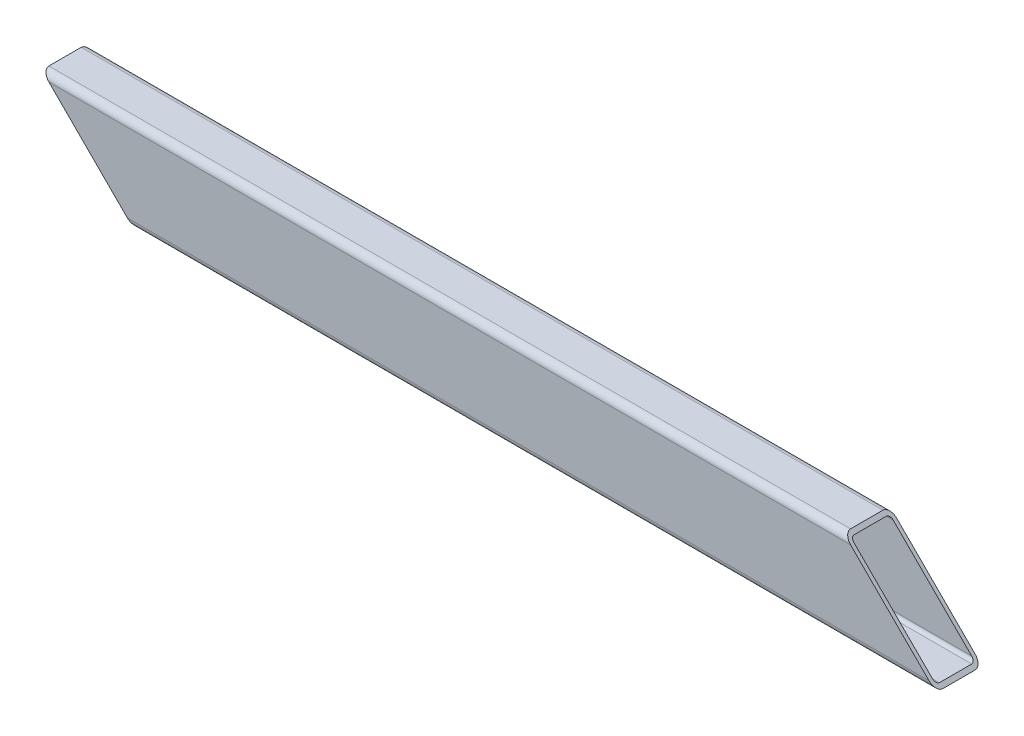
from build123d import *

# Parameters (mm, degrees)
COLD_FORMED_RECT_HOLLOW_SECTION_GB_T_672_DEPTH = 775
CUT_EXTRUDE1_DEPTH                             = 778.061773606


with BuildPart() as part:
    # Sketch1 → Cold-Formed Rect Hollow Section GB/T 6728-2002 80 X 40 X 3(1) (new body)
    with BuildSketch(Plane(origin=(0, 0, 0), x_dir=(0, 0, -1), z_dir=(1, 0, 0))):
        with BuildLine():
            Line((-14, -40), (14, -40))
            ThreePointArc((14, -40), (18.242640687, -38.242640687), (20, -34))
            Line((20, -34), (20, 34))
            ThreePointArc((20, 34), (18.242640687, 38.242640687), (14, 40))
            Line((14, 40), (-14, 40))
            ThreePointArc((-14, 40), (-18.242640687, 38.242640687), (-20, 34))
            Line((-20, 34), (-20, -34))
            ThreePointArc((-20, -34), (-18.242640687, -38.242640687), (-14, -40))
        make_face()
        with BuildLine():
            Line((-14, -37), (14, -37))
            ThreePointArc((14, -37), (16.121320344, -36.121320344), (17, -34))
            Line((17, -34), (17, 34))
            ThreePointArc((17, 34), (16.121320344, 36.121320344), (14, 37))
            Line((14, 37), (-14, 37))
            ThreePointArc((-14, 37), (-16.121320344, 36.121320344), (-17, 34))
            Line((-17, 34), (-17, -34))
            ThreePointArc((-17, -34), (-16.121320344, -36.121320344), (-14, -37))
        make_face(mode=Mode.SUBTRACT)
    extrude(amount=COLD_FORMED_RECT_HOLLOW_SECTION_GB_T_672_DEPTH)

    # Sketch2 → Cut-Extrude1 (cut, through all)
    with BuildSketch(Plane.XY.offset(20)):
        Polygon((0, 40), (80, -40), (0, -40), (0, -34), (0, 34), align=None)
        Polygon((775, 40), (695, 40), (775, -40), align=None)
    extrude(amount=-CUT_EXTRUDE1_DEPTH, mode=Mode.SUBTRACT)


solid = part.part
